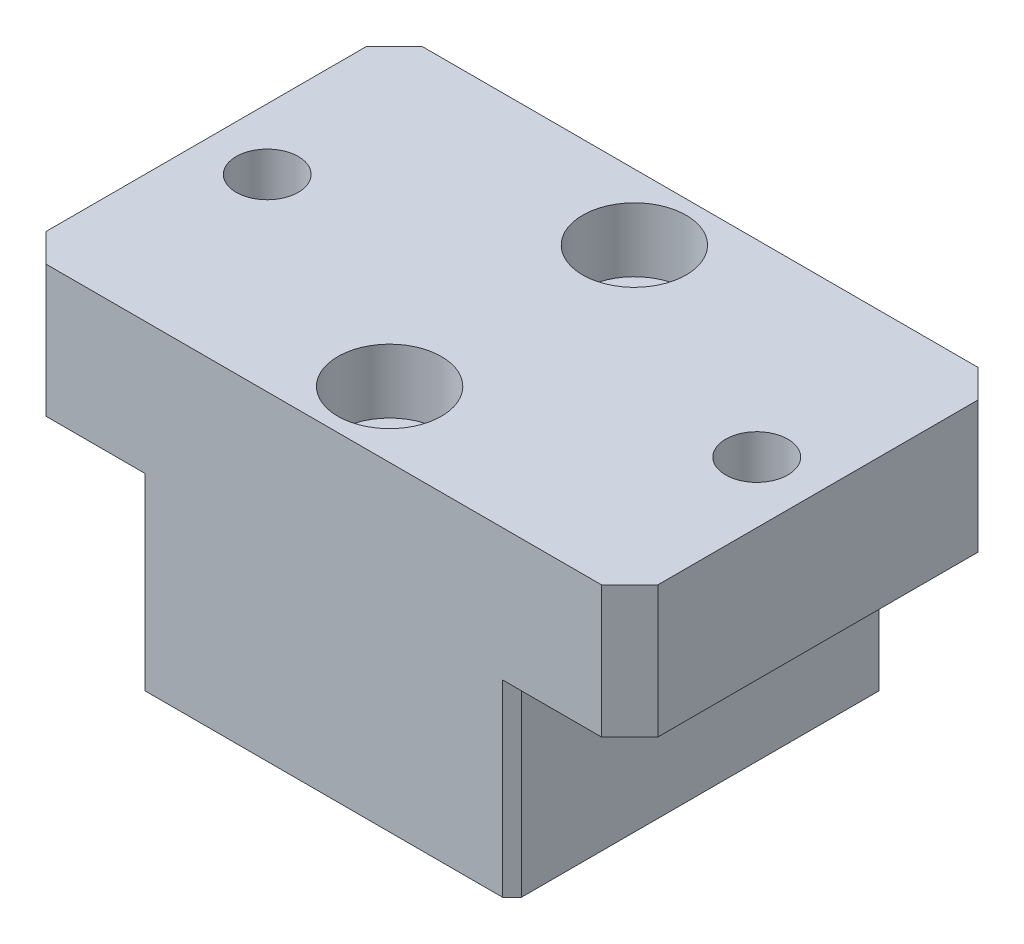
SolidWorks part; units mm, degrees
material "A6061"
ref_plane "前基準面" through (0, 0, 0) normal (0, 0, 1) x (1, 0, 0)
ref_plane "上基準面" through (0, 0, 0) normal (0, 1, 0) x (1, 0, 0)
ref_plane "右基準面" through (0, 0, 0) normal (1, 0, 0) x (0, 0, -1)
sketch "草图1" plane through (0, 0, 0) normal (0, 1, 0) x (1, 0, 0)
  line L1 (-32.5, -20) -> (32.5, -20)
  line L2 (-32.5, -20) -> (-32.5, 20)
  line L3 (-32.5, 20) -> (32.5, 20)
  line L4 (32.5, -20) -> (32.5, 20)
  line L5 (-32.5, -20) -> (32.5, 20) construction
  line L6 (-32.5, 20) -> (32.5, -20) construction
  point P0 (0, 0)
  dimension "D1" = 65
  dimension "D2" = 40
extrude "凸台-拉伸1" add sketch "草图1" along normal mid plane 34
hole_wizard "打孔尺寸(%根据)内六角圆柱头螺钉的类型2" positions "草图2" profile "草图3" counterbore size "M6" standard "GB" end condition through all
sketch "草图2" plane through (0, 17, 0) normal (0, 1, 0) x (1, 0, 0)
  line L0 (0, -33.8061) -> (0, 0) construction
  line L1 (0, 0) -> (35.081, 0) construction
  point P0 (0, -13)
  point P11 (0, 13)
  dimension "D1" = 26
sketch "草图3" plane through (0, 17, 13) normal (1, 0, 0) x (0, 0, 1)
  line L0 (0, 0) -> (0, 34)
  line L1 (0, 34) -> (3.3, 34)
  line L3 (3.3, 34) -> (3.3, 6.8)
  line L4 (3.3, 6.8) -> (5.5, 6.8)
  line L5 (5.5, 6.8) -> (5.5, 0)
  line L7 (5.5, 0) -> (0, 0)
  line L11 (0, -6.35) -> (0, 107.95) construction
  dimension "通孔孔直径" = 6.6
  dimension "通孔孔深度" = 34
  dimension "柱形沉头孔直径" = 11
  dimension "柱形沉头孔深度" = 6.8
chamfer "倒角1" distance 3 angle 45 4 edges at (32.5, 0, 20) (32.5, 0, -20) (-32.5, 0, -20) (-32.5, 0, 20)
sketch "草图6" plane through (0, -17, 0) normal (0, -1, 0) x (1, 0, 0)
  line L0 (-29.5, 20) -> (29.5, 20) construction
  line L1 (20, -20) -> (-20, -20)
  line L2 (20, -20) -> (20, 20)
  line L3 (20, 20) -> (-20, 20)
  line L4 (-20, -20) -> (-20, 20)
  line L5 (20, -20) -> (-20, 20) construction
  line L6 (20, 20) -> (-20, -20) construction
  point P0 (0, 0)
  dimension "D1" = 40
extrude "切除-拉伸1" cut sketch "草图6" against normal blind 20 flip side to cut
hole_wizard "打孔尺寸(%根据)内六角圆柱头螺钉的类型2" positions "草图4" profile "草图5" counterbore size "M6" standard "GB" end condition through all
sketch "草图4" plane through (0, 3, 0) normal (0, 1, 0) x (1, 0, 0)
  line L0 (0, -28.8438) -> (0, 0) construction
  point P0 (26, 0)
  point P8 (-26, 0)
  dimension "D1" = 52
sketch "草图5" plane through (26, 3, 0) normal (1, 0, 0) x (0, 0, -1)
  line L0 (0, 0) -> (0, 14)
  line L1 (0, 14) -> (3.3, 14)
  line L3 (3.3, 14) -> (3.3, 5)
  line L4 (3.3, 5) -> (5.5, 5)
  line L5 (5.5, 5) -> (5.5, 0)
  line L7 (5.5, 0) -> (0, 0)
  line L11 (0, -6.35) -> (0, 107.95) construction
  dimension "通孔孔直径" = 6.6
  dimension "通孔孔深度" = 14
  dimension "柱形沉头孔直径" = 11
  dimension "柱形沉头孔深度" = 5
chamfer "倒角2" distance 1 angle 45 4 edges at (-20, -7, 20) (20, -7, 20) (-20, -7, -20) (20, -7, -20)
